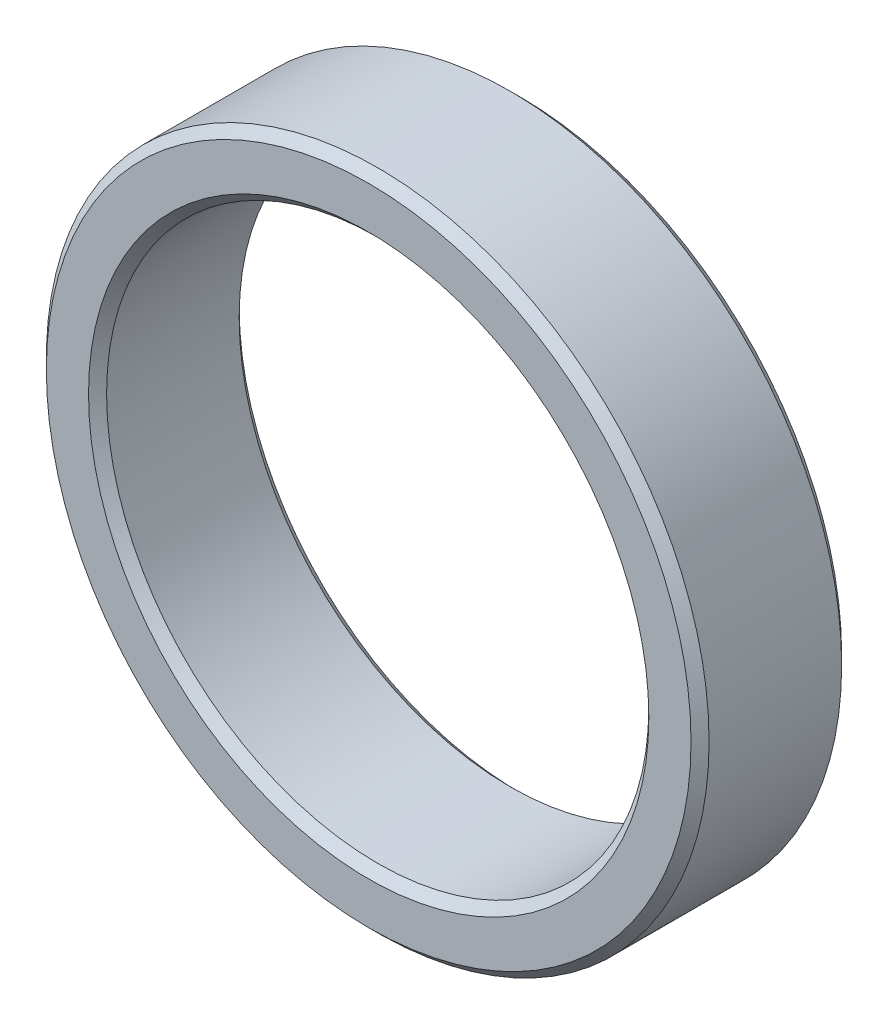
SolidWorks part; units mm, degrees
ref_plane "前视基准面" through (0, 0, 0) normal (0, 0, 1) x (1, 0, 0)
ref_plane "上视基准面" through (0, 0, 0) normal (0, 1, 0) x (1, 0, 0)
ref_plane "右视基准面" through (0, 0, 0) normal (1, 0, 0) x (0, 0, -1)
sketch "草图2" plane through (0, 0, 0) normal (0, 0, 1) x (1, 0, 0)
  circle A0 centre (0, 0) radius 11
  dimension "D1" = 22
extrude "凸台-拉伸1" add sketch "草图2" along normal blind 5
sketch "草图3" plane through (0, 0, 5) normal (0, 0, 1) x (1, 0, 0)
  circle A0 centre (0, 0) radius 9
  dimension "D1" = 18
extrude "切除-拉伸1" cut sketch "草图3" against normal blind 5
chamfer "倒角2" distance 0.3 angle 45 4 edges at (9, 0, 0) (9, 0, 5) (11, 0, 0) (11, 0, 5)
